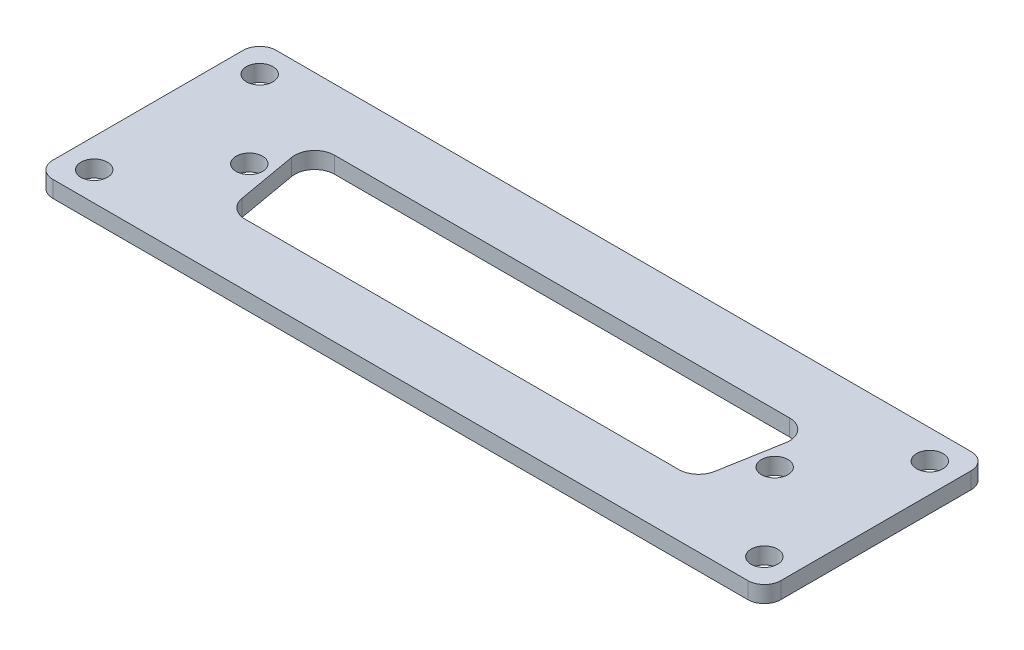
from build123d import *

# Parameters (mm, degrees)
SKETCH1_W           = 88
SKETCH1_H           = 27
BOSS_EXTRUDE1_DEPTH = 2
SKETCH2_R           = 1.6
CUT_EXTRUDE1_DEPTH  = 47.067884692
FILLET1_R           = 2
CUT_EXTRUDE2_DEPTH  = 47.067884692
M3_TAPPED_HOLE1_D   = 2.5
SKETCH6_R           = 1.6
CUT_EXTRUDE3_DEPTH  = 47.067884692


with BuildPart() as part:
    # Sketch1 → Boss-Extrude1 (new body)
    with BuildSketch(Plane(origin=(0, 0, 0), x_dir=(1, 0, 0), z_dir=(0, 1, 0))):
        Rectangle(SKETCH1_W, SKETCH1_H)
    extrude(amount=BOSS_EXTRUDE1_DEPTH)

    # Sketch2 → Cut-Extrude1 (cut, through all)
    with BuildSketch(Plane(origin=(0, 2, 0), x_dir=(1, 0, 0), z_dir=(0, 1, 0))):
        with Locations(Location((-40.5, 10, 0), (0, 0, 270))):
            Circle(SKETCH2_R)
        with Locations(Location((40.5, 10, 0), (0, 0, 270))):
            Circle(SKETCH2_R)
        with Locations(Location((40.5, -10, 0), (0, 0, 270))):
            Circle(SKETCH2_R)
        with Locations(Location((-40.5, -10, 0), (0, 0, 270))):
            Circle(SKETCH2_R)
    extrude(amount=-CUT_EXTRUDE1_DEPTH, mode=Mode.SUBTRACT)

    # Fillet1
    fillet1_edges = [part.edges().sort_by_distance(p)[0] for p in [
        (44, 1, 13.5),
        (-44, 1, 13.5),
        (-44, 1, -13.5),
        (44, 1, -13.5),
    ]]
    fillet(fillet1_edges, radius=FILLET1_R)

    # Sketch3 → Cut-Extrude2 (cut, through all)
    with BuildSketch(Plane(origin=(0, 2, 0), x_dir=(1, 0, 0), z_dir=(0, 1, 0))):
        with BuildLine():
            Line((-29.863538607, 3.233244374), (-28.576351648, -4.066755626))
            ThreePointArc((-28.576351648, -4.066755626), (-27.755503304, -5.488506663), (-26.212813041, -6.05))
            Line((-26.212813041, -6.05), (26.212813041, -6.05))
            ThreePointArc((26.212813041, -6.05), (27.755503304, -5.488506663), (28.576351648, -4.066755626))
            Line((28.576351648, -4.066755626), (29.863538607, 3.233244374))
            ThreePointArc((29.863538607, 3.233244374), (29.338506663, 5.192690263), (27.5, 6.05))
            Line((27.5, 6.05), (-27.5, 6.05))
            ThreePointArc((-27.5, 6.05), (-29.338506663, 5.192690263), (-29.863538607, 3.233244374))
        make_face()
    extrude(amount=-CUT_EXTRUDE2_DEPTH, mode=Mode.SUBTRACT)

    # M3 Tapped Hole1 (through all)
    with Locations(Plane(origin=(0, 2, 0), x_dir=(1, 0, 0), z_dir=(0, 1, 0))):
        with Locations((-31.75, 0), (31.75, 0)):
            Hole(M3_TAPPED_HOLE1_D / 2)

    # Sketch6 → Cut-Extrude3 (cut, through all)
    with BuildSketch(Plane(origin=(0, 2, 0), x_dir=(1, 0, 0), z_dir=(0, 1, 0))):
        with Locations(Location((-31.75, 0, 0), (0, 0, 270))):
            Circle(SKETCH6_R)
        with Locations(Location((31.75, 0, 0), (0, 0, 270))):
            Circle(SKETCH6_R)
    extrude(amount=-CUT_EXTRUDE3_DEPTH, mode=Mode.SUBTRACT)


solid = part.part
